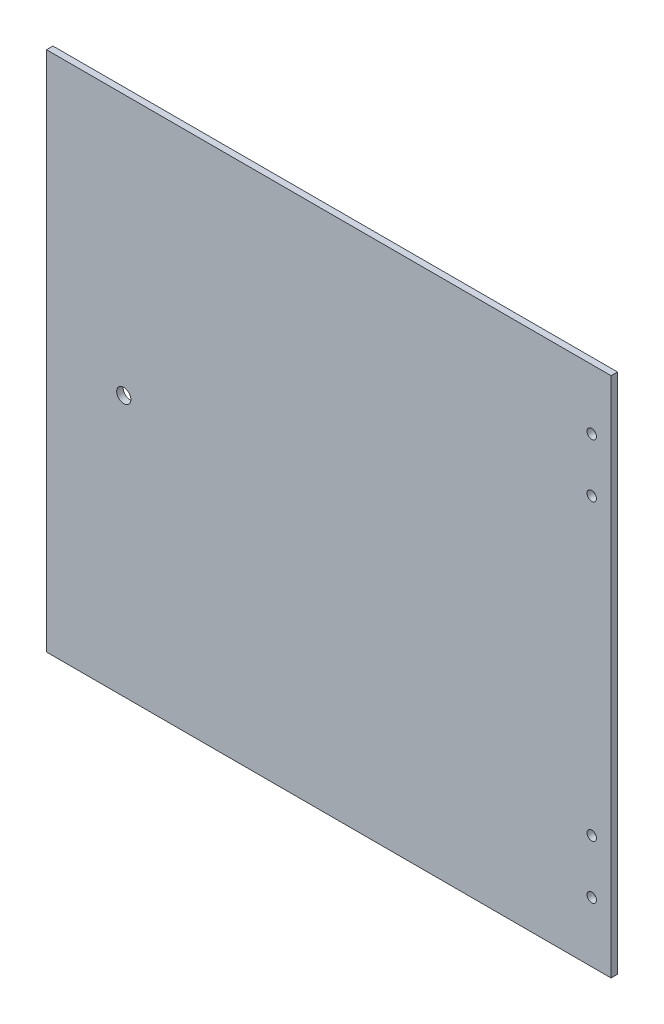
from build123d import *

# Parameters (mm, degrees)
SKETCH_1_W          = 263
SKETCH_1_H          = 243
EXTRUDE_1_DEPTH     = 3
SKETCH_4_R          = 2.2
CUT_EXTRUDE_2_DEPTH = 10
SKETCH_5_R          = 3.3
CUT_EXTRUDE_3_DEPTH = 10


with BuildPart() as part:
    # 草图1 → 凸台-拉伸1 (new body)
    with BuildSketch(Plane.XY):
        Rectangle(SKETCH_1_W, SKETCH_1_H)
    extrude(amount=EXTRUDE_1_DEPTH)

    # 草图4 → 切除-拉伸2 (cut)
    with BuildSketch(Plane(origin=(0, 0, 0), x_dir=(-1, 0, 0), z_dir=(0, 0, -1))):
        with Locations((-122.5, -68.5)):
            Circle(SKETCH_4_R)
        with Locations((-122.5, -93.5)):
            Circle(SKETCH_4_R)
    cut_extrude_2 = extrude(amount=-CUT_EXTRUDE_2_DEPTH, mode=Mode.SUBTRACT)

    # 镜向1: 切除-拉伸2 across plane
    add(cut_extrude_2.mirror(Plane.ZX), mode=Mode.SUBTRACT)

    # 草图5 → 切除-拉伸3 (cut)
    with BuildSketch(Plane.XY.offset(3)):
        with Locations((-95.5, 0)):
            Circle(SKETCH_5_R)
    extrude(amount=-CUT_EXTRUDE_3_DEPTH, mode=Mode.SUBTRACT)


solid = part.part
